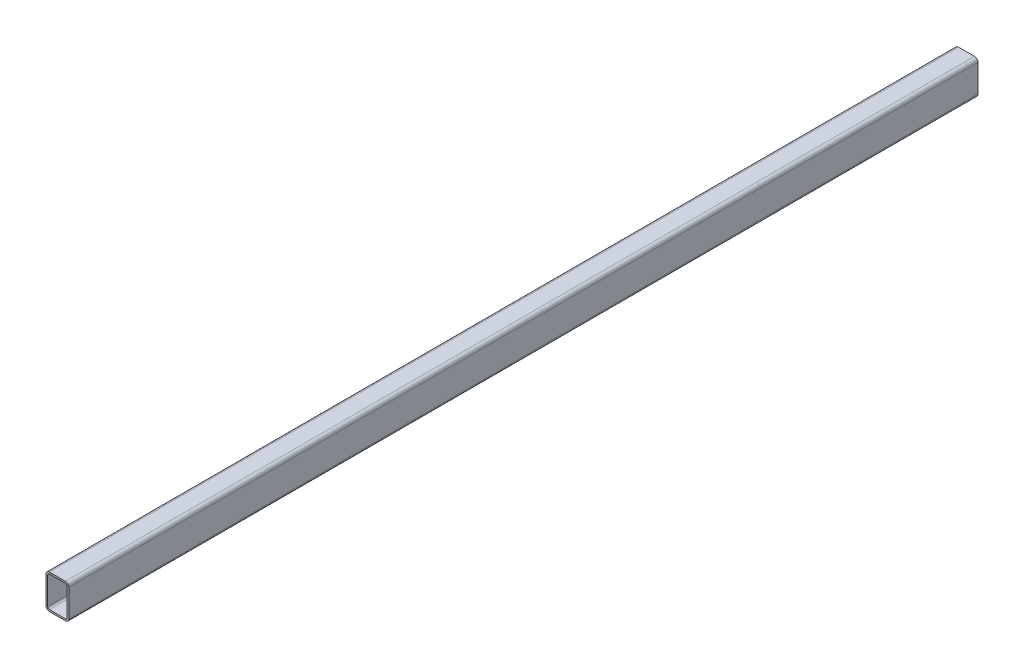
from build123d import *

# Parameters (mm, degrees)
GB_6728_1986_RECTANGULAR_HOLLOW_SECTION_DEPTH = 1590


with BuildPart() as part:
    # Sketch14 → Gb/6728-1986 rectangular hollow section 060 X 40 X 3 (new body)
    with BuildSketch(Plane(origin=(0, 0, 0), x_dir=(-1, 0, 0), z_dir=(0, 0, -1))):
        with BuildLine():
            Line((-14, -30), (14, -30))
            ThreePointArc((14, -30), (18.242640687, -28.242640687), (20, -24))
            Line((20, -24), (20, 24))
            ThreePointArc((20, 24), (18.242640687, 28.242640687), (14, 30))
            Line((14, 30), (-14, 30))
            ThreePointArc((-14, 30), (-18.242640687, 28.242640687), (-20, 24))
            Line((-20, 24), (-20, -24))
            ThreePointArc((-20, -24), (-18.242640687, -28.242640687), (-14, -30))
        make_face()
        with BuildLine():
            Line((-14, -27), (14, -27))
            ThreePointArc((14, -27), (16.121320344, -26.121320344), (17, -24))
            Line((17, -24), (17, 24))
            ThreePointArc((17, 24), (16.121320344, 26.121320344), (14, 27))
            Line((14, 27), (-14, 27))
            ThreePointArc((-14, 27), (-16.121320344, 26.121320344), (-17, 24))
            Line((-17, 24), (-17, -24))
            ThreePointArc((-17, -24), (-16.121320344, -26.121320344), (-14, -27))
        make_face(mode=Mode.SUBTRACT)
    extrude(amount=GB_6728_1986_RECTANGULAR_HOLLOW_SECTION_DEPTH)


solid = part.part
